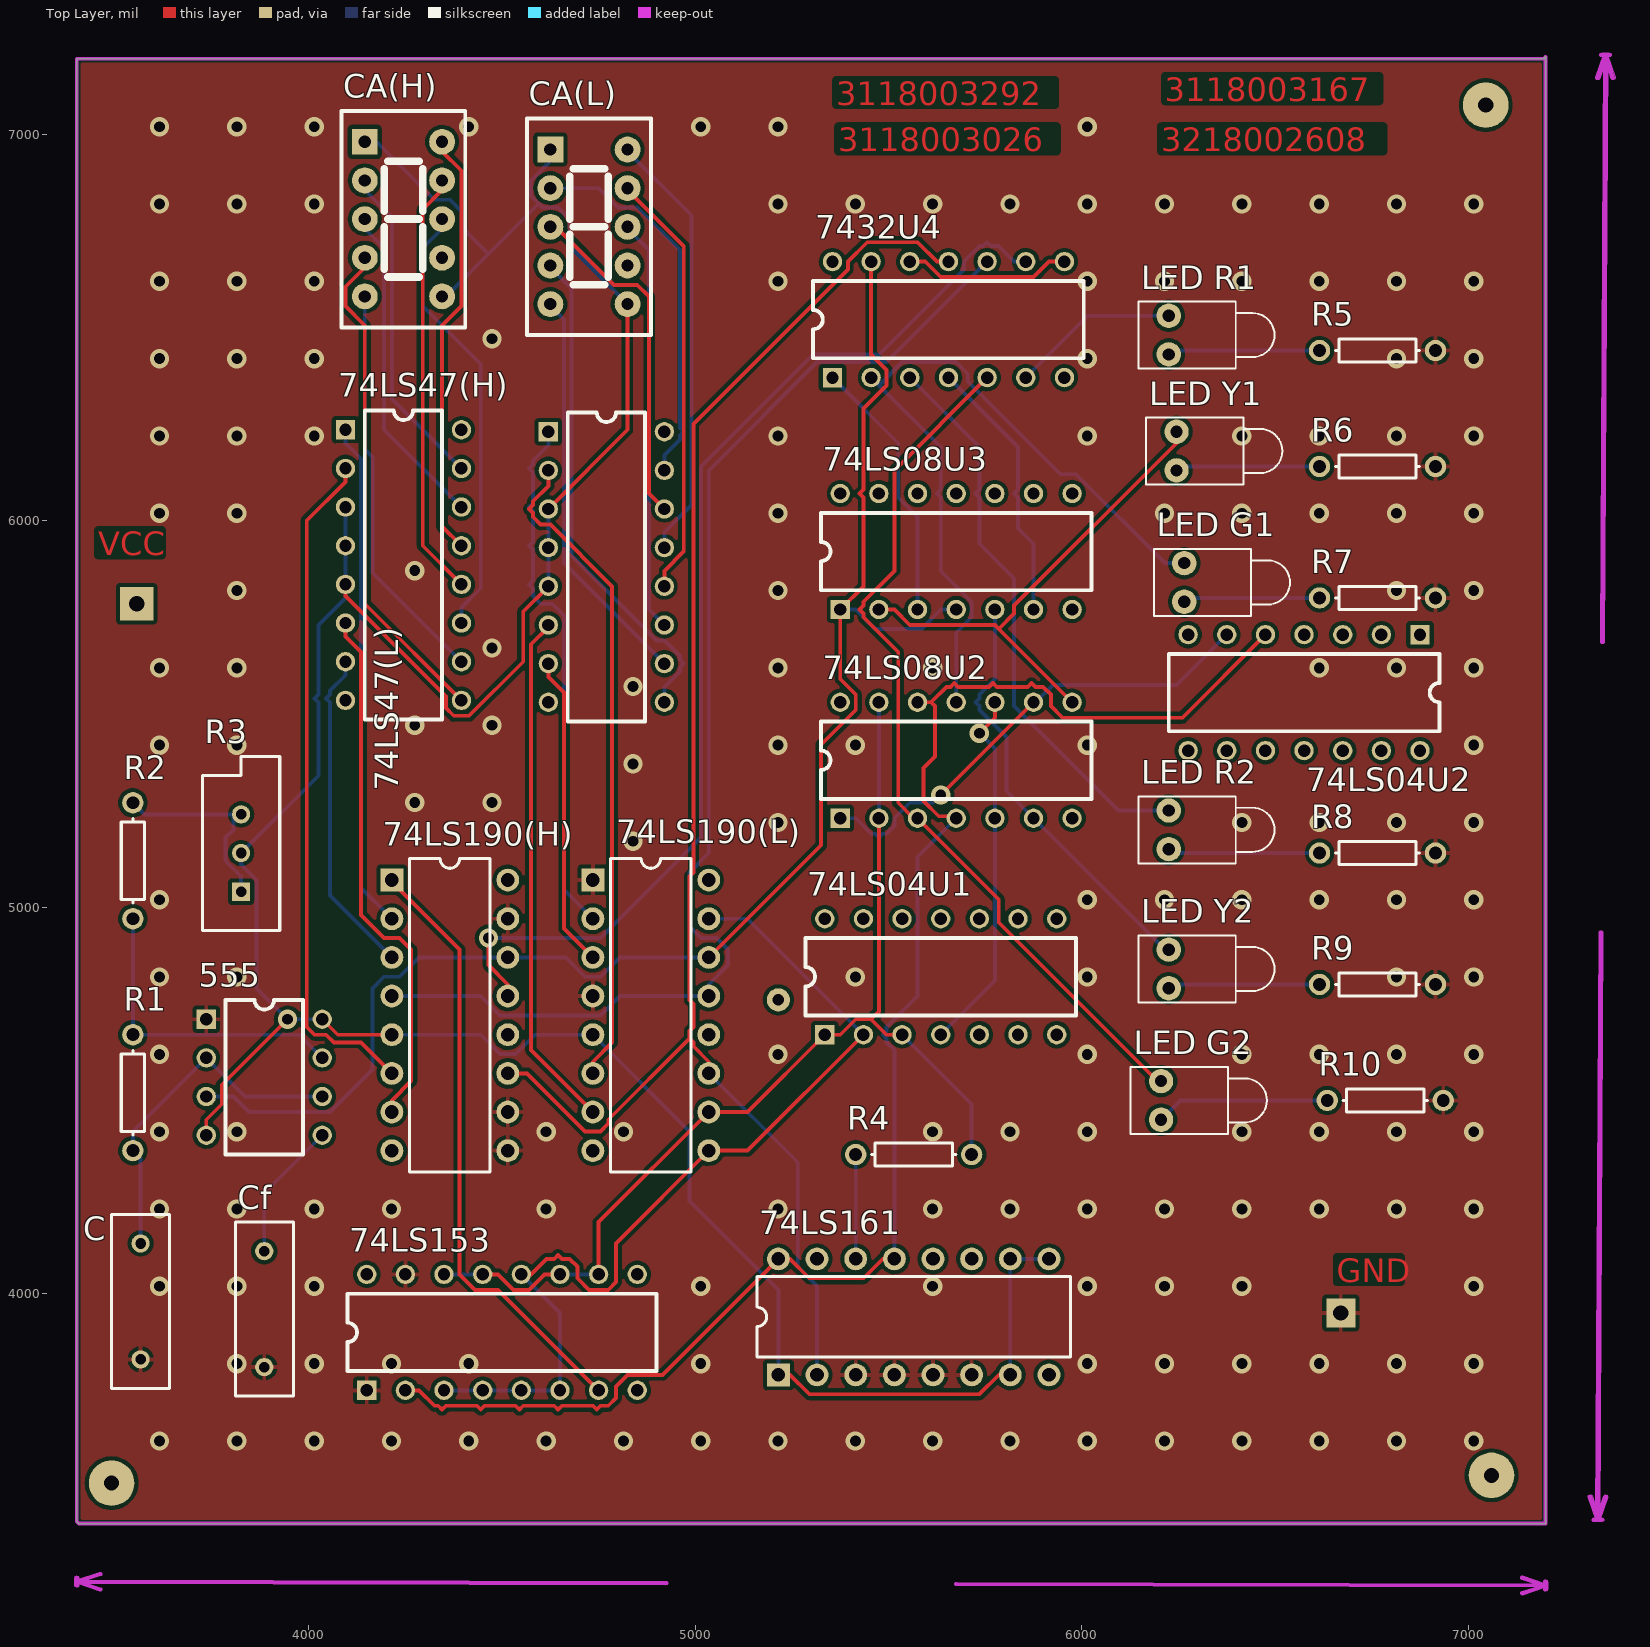
[diagram p0: Top Layer view]
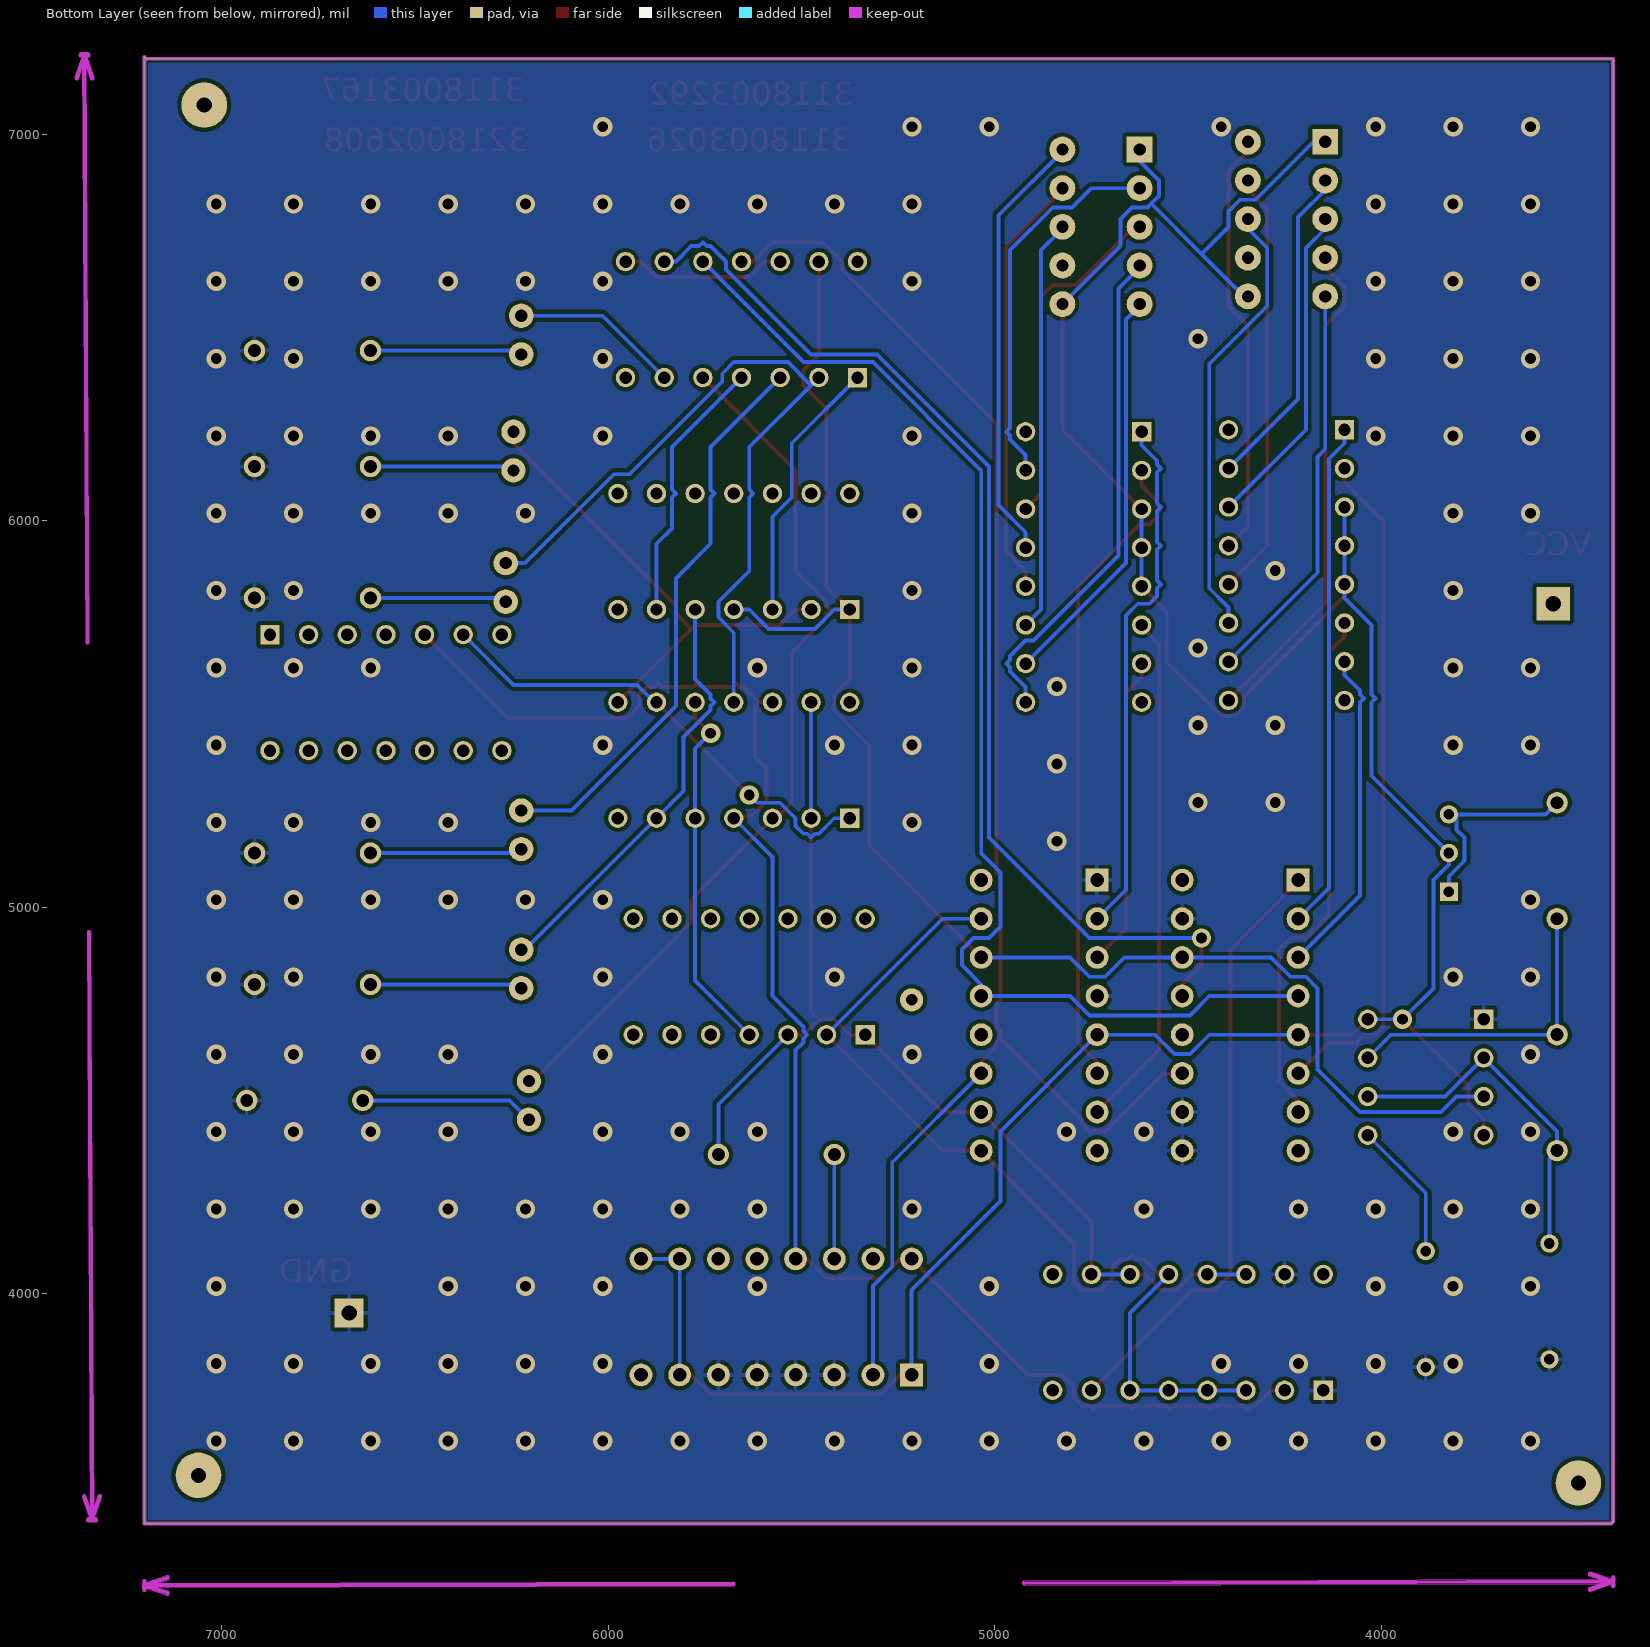
[diagram p1: Bottom Layer view, seen from below]
# Altium PCB MISC75419.pcbdoc
Units mil, origin at the board's own origin, x right, y up, seen from the top; angles counter-clockwise.
Board outline 3800 x 3795 mil, 2 copper layers (Top Layer, Bottom Layer); 32 components, 55 nets, 237 pads, 172 vias.

## Layer stack, top to bottom (the 12.6 mil dielectric is the usual default, probably not edited)
Top Solder Mask Layer: solder mask 1.4, FR-4, Dk 4.8
Top Layer: signal copper 1.4
Substrate1: surface 12.6, FR-4, Dk 4.8
Bottom Layer: signal copper 1.4
Bottom Solder Mask Layer: solder mask 1.4, FR-4, Dk 4.8

## Board outline
3400,3410 3400,7195 7195,7195 7200,7200 7200,3405 3405,3405

## Design rules (kind name [scope] priority, off if disabled: settings)
BoardOutlineClearance Plane_PlaneConnect_1 [All] p2 off: genericclearance=10 ignorepadtopadclearanceinfootprint=FALSE except(0: Arc-SplitContinuation Track-SplitContinuation SMDPad-SplitContinuation THPad-SplitContinuation Via-SplitContinuation Fill-SplitContinuation Region-SplitContinuation Poly-SplitContinuation Text-SplitContinuation Hole-SplitContinuation; 6: SMDPad-CutoutEdge THPad-CutoutEdge Via-CutoutEdge Fill-CutoutEdge Region-CutoutEdge Text-CutoutEdge; 6.9: Hole-CutoutEdge; 10: Arc-OutlineEdge Track-OutlineEdge SMDPad-OutlineEdge THPad-OutlineEdge Via-OutlineEdge Fill-OutlineEdge Region-OutlineEdge Poly-OutlineEdge Text-OutlineEdge Hole-OutlineEdge Poly-CutoutEdge; 11.8: Arc-CutoutEdge Track-CutoutEdge)
BoardOutlineClearance Copper_PolygonConnect_1 [All] p4 off: genericclearance=10 ignorepadtopadclearanceinfootprint=FALSE except(0: Arc-SplitContinuation Track-SplitContinuation SMDPad-SplitContinuation THPad-SplitContinuation Via-SplitContinuation Fill-SplitContinuation Region-SplitContinuation Poly-SplitContinuation Text-SplitContinuation Hole-SplitContinuation; 6: SMDPad-CutoutEdge THPad-CutoutEdge Via-CutoutEdge Fill-CutoutEdge Region-CutoutEdge Text-CutoutEdge; 6.9: Hole-CutoutEdge; 10: Arc-OutlineEdge Track-OutlineEdge SMDPad-OutlineEdge THPad-OutlineEdge Via-OutlineEdge Fill-OutlineEdge Region-OutlineEdge Poly-OutlineEdge Text-OutlineEdge Hole-OutlineEdge Poly-CutoutEdge; 11.8: Arc-CutoutEdge Track-CutoutEdge)
BoardOutlineClearance Clearance_1 [All] p6: genericclearance=10 ignorepadtopadclearanceinfootprint=FALSE except(0: Arc-SplitContinuation Track-SplitContinuation SMDPad-SplitContinuation THPad-SplitContinuation Via-SplitContinuation Fill-SplitContinuation Region-SplitContinuation Poly-SplitContinuation Text-SplitContinuation Hole-SplitContinuation; 6: SMDPad-CutoutEdge THPad-CutoutEdge Via-CutoutEdge Fill-CutoutEdge Region-CutoutEdge Text-CutoutEdge; 6.9: Hole-CutoutEdge; 10: Arc-OutlineEdge Track-OutlineEdge SMDPad-OutlineEdge THPad-OutlineEdge Via-OutlineEdge Fill-OutlineEdge Region-OutlineEdge Poly-OutlineEdge Text-OutlineEdge Hole-OutlineEdge Poly-CutoutEdge; 11.8: Arc-CutoutEdge Track-CutoutEdge)
Clearance Plane_PlaneConnect [All] p1 off: gap=10 ignorepadtopadclearanceinfootprint=FALSE
Clearance Copper_PolygonConnect [All] p3 off: gap=10 ignorepadtopadclearanceinfootprint=FALSE
Clearance [All] p5: gap=10 ignorepadtopadclearanceinfootprint=FALSE
DiffPairsRouting [All] p1: maxlimit=10 minlimit=10 mostfreqgap=10 toplayer_minwidth=0 toplayer_prefwidth=0 toplayer_maxwidth=0 toplayer_mingap=10 toplayer_prefgap=10 toplayer_maxgap=10 bottomlayer_minwidth=0 bottomlayer_prefwidth=0 bottomlayer_maxwidth=0 bottomlayer_mingap=10 bottomlayer_prefgap=10 bottomlayer_maxgap=10 maxuncoupledlength=10
HoleToHoleClearance ComponentClearance [All] p1: gap=10 allowstackedmicrovias=TRUE
Length netLength [All] p1: minlimit=0 maxlimit=0
PolygonConnect [(InNet('GND'))] p1: connectstyle=Relief reliefconductorwidth=10 reliefentries=4 polygonreliefangle="90 Angle" airgapwidth=10 via.connectstyle=Relief via.reliefconductorwidth=10 via.reliefentries=4 via.polygonreliefangle="90 Angle" via.airgapwidth=10
RoutingVias [All] p1: holewidth=28 width=50 viastyle="Through Hole" minholewidth=28 minwidth=50 maxholewidth=28 maxwidth=50
SolderMaskExpansion [All] p1: expansion=4 istentingtop=FALSE
Width [All] p1: maxlimit=10 minlimit=10 preferedwidth=10
2 further rules are at their usual default settings.

## Components (designator, comment, footprint, x,y, rotation, side; value= is the part's Value field where it differs from the comment)
74LS04U1 "74LS04" DIP14 5985,4720 r90 top
74LS04U2 "74LS04" DIP14 6225,5655 r270 top
74LS08U2 "74LS08" DIP14 6025,5280 r90 top
74LS08U3 "74LS08" DIP14 6025,5820 r90 top
74LS47(H) "SN7447A" DIP16 4145,5480 r0 top
74LS47(L) "SN7447A" DIP16 4670,5475 r0 top
74LS153 "SN74LS153" DIP16 4905,3800 r90 top
74LS161 "74LS161A" DIP-16 5565,3940 r0 top
74LS190(H) "SN74LS190" DIP-16 4365,4720 r270 top
74LS190(L) "SN74LS190" DIP-16 4885,4720 r270 top
555 "555" DIP8 3785,4360 r0 top
7432U4 "7432" DIP14 6005,6420 r90 top
C "Cap" RAD-0.3 3565,3980 r90 top
CA(H) "Dpy Red-CA" "SMG 0.36-1P" 4245,6780 r0 top
CA(L) "Dpy Red-CA" "SMG 0.36-1P" 4725,6760 r0 top
Cf "Cap" RAD-0.3 3885,3960 r90 top
"LED G1" "LED1" LED-1 6265,5840 r0 top
"LED G2" "LED1" LED-1 6205,4500 r0 top
"LED R1" "LED1" LED-1 6225,6480 r0 top
"LED R2" "LED1" LED-1 6225,5200 r0 top
"LED Y1" "LED1" LED-1 6245,6180 r0 top
"LED Y2" "LED1" LED-1 6225,4840 r0 top
R1 "Res1" AXIAL-0.3 3545,4520 r90 top
R2 "Res1" AXIAL-0.3 3545,5120 r90 top
R3 "RPot" VR5 3825,5140 r90 top
R4 "Res1" AXIAL-0.3 5565,4360 r180 top
R5 "Res1" AXIAL-0.3 6765,6440 r0 top
R6 "Res1" AXIAL-0.3 6765,6140 r0 top
R7 "Res1" AXIAL-0.3 6765,5800 r0 top
R8 "Res1" AXIAL-0.3 6765,5140 r0 top
R9 "Res1" AXIAL-0.3 6765,4800 r0 top
R10 "Res1" AXIAL-0.3 6785,4500 r0 top

## Footprints (in the part's own frame and the unit in brackets; to place one, negate y for a bottom-side part, rotate by r counter-clockwise, add the part's x,y. Pads: shape width x height; smd on the part's side, far side on the other; paste and mask are expansions set on the pad)
AXIAL-0.3 [mm]
  round 1.4 hole 0.85: 1(-3.81,0) 2(3.81,0)
  silkscreen extent -2.77,-0.76 2.77,0.76
DIP8 [mil]
  rect 50x50 hole 32: 1(-50,350)
  round 50 hole 32: 2(-50,250) 3(-50,150) 4(-50,50) 5(250,50) 6(250,150) 7(250,250) 8(250,350)
  silkscreen extent 0,0 200,400
DIP14 [mil]
  rect 50x50 hole 32: 1(-50,650)
  round 50 hole 32: 2(-50,550) 3(-50,450) 4(-50,350) 5(-50,250) 6(-50,150) 7(-50,50) 8(250,50) 9(250,150) 10(250,250) 11(250,350) 12(250,450) 13(250,550) 14(250,650)
  silkscreen extent 0,0 200,700
DIP16 [mil]
  rect 50x50 hole 32: 1(-50,755)
  round 50 hole 32: 2(-50,655) 3(-50,555) 4(-50,455) 5(-50,355) 6(-50,255) 7(-50,155) 8(-50,55) 9(250,55) 10(250,155) 11(250,255) 12(250,355) 13(250,455) 14(250,555) 15(250,655) 16(250,755)
  silkscreen extent 0,5 200,805
DIP-16 [mm]
  rect 1.5x1.5 hole 0.9: 1(-8.89,-3.81)
  round 1.5 hole 0.9: 2(-6.35,-3.81) 3(-3.81,-3.81) 4(-1.27,-3.81) 5(1.27,-3.81) 6(3.81,-3.81) 7(6.35,-3.81) 8(8.89,-3.81) 9(8.89,3.81) 10(6.35,3.81) 11(3.81,3.81) 12(1.27,3.81) 13(-1.27,3.81) 14(-3.81,3.81) 15(-6.35,3.81) 16(-8.89,3.81)
  silkscreen extent -10.3,-2.65 10.3,2.65
LED-1 [mm]
  round 1.6 hole 0.8: 1(0,1.27) 2(0,-1.27)
  silkscreen extent -2,-2.2 6.95,2.2
RAD-0.3 [mm]
  round 1.2 hole 0.7: 1(-3.81,0) 2(3.81,0)
  silkscreen extent -5.71,-1.91 5.71,1.91
"SMG 0.36-1P" [mm]
  rect 1.7x1.7 hole 0.8: 1(-2.54,5.08)
  round 1.7 hole 0.8: 2(-2.54,2.54) 3(-2.54,0) 4(-2.54,-2.54) 5(-2.54,-5.08) 6(2.54,-5.08) 7(2.54,-2.54) 8(2.54,0) 9(2.54,2.54) 10(2.54,5.08)
  silkscreen extent -4.06,-7.11 4.06,7.11
VR5 [mm]
  rect 1.2x1.2 hole 0.7: 1(-2.54,0)
  round 1.2 hole 0.7: 2(0,0) 3(2.54,0)
  silkscreen extent -5.08,-2.54 6.35,2.54

## Free pads (board coordinates)
  round 60 hole 30 paste+0 mask+4: 1(5215,4760)
  rect 86.61x86.61 hole 39.37 paste+0 mask+4: 2(3555,5785)
  rect 74.8x74.8 hole 39.37 paste+0 mask+4: 3(6670,3950)
  round 118.11 hole 39.37 unplated paste-1000 mask+4: 12(3490,3510) 12(7045,7075) 12(7060,3530)

## Via types
v1: diameter 50, hole 28, Top Layer to Bottom Layer, 172 vias

## Nets (pads, with @x,y where several pads share a name; then routed paths per layer and width w, separated by ;. In a path a pad name is that pad's centre, name@x,y a point inside that pad or via, vN(x,y) a via of type N, cw(c..) or ccw(c..) an arc to the next point about the centre after c; other vN are vias at no path point)
$2N11: 74LS47(H).13 CA(H).10 | length 1107.1
  Top Layer w10: 4345,6980 4345,6955 4395,6905 4395,6555 4345,6505 4345,5985 4395,5935
$2N12: 74LS47(H).12 CA(H).9 | length 1107.1
  Top Layer w10: 4345,6880 4345,6855 4295,6805 4295,5935 4395,5835
$2N13: 74LS47(H).11 CA(H).8 | length 1148.6
  Bottom Layer w10: 4345,6780 4345,6755 4295,6705 4295,6555 4445,6405 4445,5825 4395,5775 4395,5735
$2N14: 74LS47(H).10 CA(H).5 | length 1048.6
  Bottom Layer w10: 4145,6580 4145,6185 4165,6165 4165,5865 4395,5635
$2N15: 74LS47(H).9 CA(H).4 | length 1290
  Top Layer w10: 4145,6680 4145,6655 4095,6605 4095,6555 4145,6505 4145,5785 4395,5535
$2N16: 74LS47(H).15 CA(H).2 | length 848.6
  Bottom Layer w10: 4145,6880 4145,6855 4215,6785 4215,6315 4395,6135
$2N17: 74LS47(H).14 CA(H).3 | length 848.6
  Bottom Layer w10: 4145,6780 4145,6755 4195,6705 4195,6235 4395,6035
$2N18: 74LS47(L).13 CA(L).10 | length 1127.3
  Bottom Layer w10: 4825,6960 4825,6955 4990,6790 4990,6040 4920,5970 4920,5930
$2N19: 74LS47(L).12 CA(L).9 | length 1110.8
  Top Layer w10: 4825,6860 4825,6855 4970,6710 4970,5920 4920,5870 4920,5830
$2N20: 74LS47(L).11 CA(L).8 | length 1069.3
  Bottom Layer w10: 4825,6760 4825,6755 4880,6700 4880,5770 4920,5730
$2N21: 74LS47(L).10 CA(L).5 | length 1052.2
  Bottom Layer w10: 4625,6560 4625,6555 4660,6520 4660,5890 4920,5630
$2N22: 74LS47(L).9 CA(L).4 | length 1305.3
  Bottom Layer w10: 4625,6660 4625,6655 4680,6600 4680,5910 4900,5690 4920,5690 4960,5650 4960,5640 4970,5630 4960,5620 4960,5610 4920,5570 4920,5530
$2N23: 74LS47(L).15 CA(L).2 | length 996.1
  Bottom Layer w10: 4625,6860 4750,6860 4800,6810 4850,6810 4960,6700 4960,6240 4970,6230 4960,6220 4960,6210 4920,6170 4920,6130
$2N24: 74LS47(L).14 CA(L).3 | length 896.1
  Top Layer w10: 4625,6760 4640,6760 4790,6610 4850,6610 4880,6580 4880,6070 4920,6030
$2N25: 74LS47(H).6 74LS190(H).7 | length 1379.6
  Top Layer w10: 4095,5735 4095,5700 4135,5660 4135,4980 4195,4920 4235,4920 4265,4890 4265,4550 4215,4500 4215,4470
$2N26: 74LS47(H).2 74LS190(H).6 | length 1756.1
  Top Layer w10: 4095,6135 4095,6100 3995,6000 3995,4690 4015,4670 4045,4670 4065,4650 4135,4650 4215,4570
$2N27: 74LS47(H).1 74LS190(H).2 | length 1314.7
  Bottom Layer w10: 4095,6235 4095,6200 4135,6160 4135,5050 4215,4970
$2N28: 74LS47(H).7 74LS190(H).3 | length 856.1
  Bottom Layer w10: 4095,5635 4095,5600 4055,5560 4055,5550 4045,5540 4055,5530 4055,5030 4215,4870
$2N29: 74LS47(L).6 74LS190(L).7 | length 1344.9
  Top Layer w10: 4620,5730 4620,5725 4575,5680 4575,4630 4735,4470
$2N30: 74LS47(L).2 74LS190(L).6 | length 1705.1
  Top Layer w10: 4620,6130 4620,6090 4580,6050 4580,6040 4570,6030 4580,6020 4580,6010 4600,5990 4625,5990 4785,5830 4785,4650 4735,4600 4735,4570
$2N31: 74LS47(L).1 74LS190(L).2 | length 1391.5
  Bottom Layer w10: 4620,6230 4620,6195 4580,6155 4580,6145 4570,6135 4580,6125 4580,6045 4570,6035 4580,6025 4580,5945 4570,5935 4580,5925 4580,5845 4570,5835 4580,5825 4580,5805 4600,5785 4630,5785 4660,5755 4660,5045 4735,4970
$2N32: 74LS47(L).7 74LS190(L).3 | length 807.6
  Top Layer w10: 4620,5630 4620,5595 4660,5555 4660,4945 4735,4870
$2N33: 74LS190(H).13 7432U4.9 | length 2901.1
  Top Layer w10: v1(4465,4920) 4465,4850 4515,4800 4515,4770
  Bottom Layer w10: v1(4465,4920) 4755,4920 5015,5180 5015,6140 5305,6430 5475,6430 5695,6650 5695,6670 5735,6710 5745,6710 5755,6720 5765,6710 5785,6710 5825,6670 7432U4.9
$2N34: 74LS190(H).4 74LS190(L).13 7432U4.10 | length 3271.4
  Bottom Layer w10: 4215,4770 4445,4770 4495,4720 4755,4720 4805,4770 5035,4770 5035,4800 5085,4850 5085,4890 5055,4920 5015,4920 4985,4950 4985,5090 5035,5140 5035,6130 5315,6410 5495,6410 7432U4.10
$2N35: 555.5 Cf.2 | length 362.1
  Bottom Layer w10: Cf.2 3885,4260 555.5
$2N36: R2.2 R3.1 R3.3 | length 517.3
  Bottom Layer w10: R2.2 3575,5240 R3.3@3805,5240 ; R3.1 3825,5080 3785,5120 3785,5180 3805,5200 R3.3@3805,5240 ; R3.3 R3.3@3805,5240
$2N37: 555.7 R1.2 R2.1 | length 814.9
  Bottom Layer w10: R2.1 R1.2 3975,4670 555.7
$2N38: 555.2 555.6 C.2 R1.1 | length 908.4
  Bottom Layer w10: C.2 3565,4350 R1.1 3545,4420 555.2 3835,4510 555.6
$2N39: 74LS153.7 74LS190(H).1 | length 1576.7
  Top Layer w10: 4215,5070 4215,5065 4390,4890 4390,4050 4430,4010 4490,4010 74LS153.7
$2N41: 74LS161.14 R4.2 | length 270
  Bottom Layer w10: 74LS161.14 R4.2
$2N45: "LED R1.2" R5.1 | length 394.1
  Bottom Layer w10: 6225,6430 6235,6440 R5.1
$2N46: "LED Y1.2" R6.1 | length 374.1
  Bottom Layer w10: 6245,6130 6255,6140 R6.1
$2N47: "LED G1.2" R7.1 | length 354.1
  Bottom Layer w10: 6265,5790 6275,5800 R7.1
$2N48: "LED R2.2" R8.1 | length 394.1
  Bottom Layer w10: 6225,5150 6235,5140 R8.1
$2N49: "LED Y2.2" R9.1 | length 394.1
  Bottom Layer w10: 6225,4790 6235,4800 R9.1
$2N50: "LED G2.2" R10.1 | length 450.7
  Bottom Layer w10: 6205,4450 6255,4500 R10.1
$2N51: 7432U4.3 "LED R2.1" | length 1482
  Bottom Layer w10: 7432U4.3 5735,6190 5735,6080 5725,6070 5735,6060 5735,5940 5825,5850 5825,5520 6095,5250 6225,5250
$2N54: 74LS08U3.1 74LS08U3.4 74LS190(H).14 74LS190(L).14 555.3 7432U4.13 | length 4036.6
  Top Layer w10: 5035,4870 5325,5160 5325,5420 5415,5510 5415,5550 5375,5590 74LS08U3.1 5435,5830 5435,6060 5425,6070 5435,6080 5435,6290 5495,6350 5495,6390 5455,6430 7432U4.13
  Bottom Layer w10: 555.3 3805,4510 3845,4470 4055,4470 4165,4580 4165,4790 4195,4820 4235,4820 4285,4870 4515,4870 4665,4870 4715,4820 4755,4820 4805,4870 5035,4870 ; 74LS08U3.1 5415,5770 5465,5720 5585,5720 5635,5770 74LS08U3.4
$2N55: 74LS08U2.6 74LS08U3.5 "LED Y2.1" | length 1113.7
  Bottom Layer w10: 74LS08U3.5 5775,5590 5735,5550 5735,5540 5725,5530 5735,5520 5735,5510 5805,5440 5805,5300 74LS08U2.6 6215,4890 6225,4890
$2N56: 7432U4.6 "LED R1.1" | length 436.3
  Bottom Layer w10: 7432U4.6 6015,6530 6225,6530
$2N57: 74LS08U3.6 7432U4.4 | length 699.4
  Bottom Layer w10: 7432U4.4 5835,6190 5835,6080 5825,6070 5835,6060 5835,5980 5875,5940 74LS08U3.6
$2N58: 74LS08U2.3 7432U4.5 "LED G2.1" | length 2291.5
  Top Layer w10: 7432U4.5 5515,6130 5515,5870 5435,5790 5435,5780 5425,5770 5435,5760 5435,5750 5525,5660 5525,5270 5565,5230 74LS08U2.3 5785,5020 5785,4960 6195,4550 6205,4550
$2N62: 7432U4.8 7432U4.12 | length 433.1
  Top Layer w10: 7432U4.12 5595,6670 5635,6630 5875,6630 5915,6670 7432U4.8
$2N63: 74LS161.2 74LS190(H).11 74LS190(L).11 7432U4.11 | length 4133.6
  Top Layer w10: 4515,4570 4565,4570 4715,4420 4755,4420 4775,4440 4775,4450 4985,4660 ; 5035,4570 5035,4600 4995,4640 4995,4650 4985,4660 ; 7432U4.11 5625,6670 5575,6720 5445,6720 5395,6670 5395,6650 4995,6250 4995,5090 4985,5080 4985,4760 4995,4750 4995,4690 4985,4680 4985,4660
  Bottom Layer w10: 5035,4570 5265,4340 5265,4070 5315,4020 74LS161.2
$2N1237: 74LS08U3.3 7432U4.1 | length 691.1
  Bottom Layer w10: 7432U4.1 5525,6200 5525,6060 5575,6010 74LS08U3.3
$2N1241: 74LS08U2.11 7432U4.2 "LED G1.1" | length 2014.5
  Bottom Layer w10: 7432U4.2 5475,6350 ; 74LS08U2.11 5675,5710 5715,5750 5715,5790 5635,5870 5635,6060 5625,6070 5635,6080 5635,6190 5475,6350 ; 6265,5890 6215,5890 5985,6120 5945,6120 5705,6360 5705,6380 5675,6410 5535,6410 5475,6350
$2N1342: 74LS04U1.4 74LS08U2.5 74LS08U2.10 | length 951.1
  Top Layer w10: v1(5735,5450) 5775,5490 74LS08U2.10
  Bottom Layer w10: 74LS04U1.4 5775,4810 74LS08U2.5 5775,5410 v1(5735,5450)
$2N1374: 74LS04U2.5 74LS08U2.4 74LS08U2.12 74LS153.2 74LS161.13 74LS161.16 | length 4226.9
  Top Layer w10: 74LS153.2 4285,3750 4325,3710 4335,3710 4345,3700 4355,3710 4435,3710 4445,3700 4455,3710 4535,3710 4545,3700 4555,3710 4635,3710 4645,3700 4655,3710 4735,3710 4745,3700 4755,3710 4775,3710 4795,3730 4795,3760 4825,3790 4915,3790 74LS161.16 5245,4090 5295,4040 5435,4040 5485,4090 74LS161.13 ; 74LS08U2.12 5610,5530 ; 74LS08U2.4 5670,5235 5630,5235 5590,5275 5590,5360 5620,5390 5620,5520 5610,5530 ; 74LS04U2.5 6259.99,5490 5949.99,5490 5919.99,5520 5919.99,5550 5899.99,5570 5880,5570 5870,5580 5860,5570 5780,5570 5770,5580 5760,5570 5680,5570 5670,5580 5660,5570 5650,5570 5610,5530
  Bottom Layer w10: 74LS161.13 5515,4630 5495,4650 5495,4660 5485,4670 5495,4680 5495,4690 5575,4770 5575,5130 74LS08U2.4
$2N1447: 74LS04U2.6 74LS08U2.1 74LS08U2.9 | length 1249.9
  Top Layer w10: v1(5635,5290) 74LS08U2.9
  Bottom Layer w10: 74LS08U2.1 5415,5230 5455,5190 5465,5190 5475,5180 5485,5190 5495,5190 5515,5210 5515,5230 5555,5270 5615,5270 v1(5635,5290) ; 74LS08U2.9 5880,5530 5925,5575 6245,5575 74LS04U2.6
$2N1530: 74LS08U2.8 74LS08U3.2 "LED Y1.1" | length 1300
  Top Layer w10: 74LS08U3.2 5515,5770 5555,5730 5775,5730 5785,5720 ; 74LS08U2.8 5785,5720 ; 6245,6230 6245,6200 5825,5780 5825,5760 5785,5720
$2N1733: 74LS04U1.2 74LS153.3 74LS153.4 74LS153.5 74LS153.6 74LS153.12 74LS190(L).9 74LS190(L).15 | length 2458.2
  Top Layer w10: 74LS153.12 4575,4050 4615,4090 4635,4090 4645,4100 4655,4090 4675,4090 4695,4070 4695,4040 4725,4010 4775,4010 4795,4030 4795,4130 5035,4370 5135,4370 74LS04U1.2
  Bottom Layer w10: 74LS153.3 74LS153.4 74LS153.5 74LS153.6 4650,3950 74LS153.12 ; 5035,4970 5135,4970 74LS04U1.2
$2N2029: 74LS04U1.1 74LS04U1.3 74LS08U2.2 74LS08U2.13 74LS153.10 74LS153.11 74LS153.13 74LS153.14 74LS190(L).10 R4.1 | length 2800
  Top Layer w10: 74LS153.13 4490,4050 4530,4010 4570,4010 4610,4050 74LS153.11 ; 74LS153.10 4750,4185 5035,4470 5135,4470 74LS04U1.1 5375,4670 5415,4710 5455,4710 ; 74LS08U2.2 5475,4730 5455,4710 ; 74LS04U1.3 5495,4670 5455,4710
  Bottom Layer w10: 74LS153.14 74LS153.13 ; 74LS153.11 74LS153.10 ; 74LS08U2.2 74LS08U2.13 ; 74LS04U1.3 5715,4490 R4.1
+5: 74LS47(H).3 74LS47(H).4 74LS47(H).5 74LS47(L).3 74LS47(L).4 74LS47(L).5 74LS161.1 74LS161.7 74LS161.9 74LS161.10 74LS190(H).5 74LS190(L).5 555.4 555.8 CA(H).1 CA(H).6 CA(L).1 CA(L).6 R3.2 | length 7941.5
  Top Layer w10: 555.4 3735,4450 3775,4490 3775,4540 v1(3945,4710) ; 555.8 4075,4670 4215,4670 ; 4095,5835 4095,5805 4355,5545 4355,5515 4375,5495 4415,5495 4555,5635 4555,5765.05 4620,5830 ; 4620,6030 4825,6235 4825,6560 ; 74LS161.1 5245,3790 5295,3740 5735,3740 5785,3790 74LS161.7
  Bottom Layer w10: 555.8 v1(3945,4710) 3865,4790 3865,5070 3825,5110 R3.2 4025,5340 4025,5530 4015,5540 4025,5550 4025,5730 4095,5800 4095,5835 4095,5935 4095,6035 ; 4145,6980 4175,6980 4325,6830 4365,6830 4395,6800 4395,6760 4465,6690 ; 4215,4670 4445,4670 4495,4620 4535,4620 4585,4670 4735,4670 4985,4420 4985,4240 5215,4010 74LS161.1 ; 4345,6580 4355,6580 4465,6690 ; 4620,5830 4620,5930 4620,6030 ; 4625,6960 4625,6930 4575,6880 4575,6840 4595,6820 ; 4825,6560 4675,6710 4675,6780 4645,6810 4605,6810 4595,6820 ; 74LS161.7 74LS161.10 74LS161.9 ; 4465,6690 4595,6820
GND: 74LS153.1 74LS153.15 74LS161.3 74LS161.4 74LS161.5 74LS161.6 74LS190(H).9 74LS190(H).10 74LS190(H).15 74LS190(L).1 74LS190(L).4 555.1 C.1 Cf.1 pad.3 R5.2 R6.2 R7.2 R8.2 R9.2 R10.2
  other v1: 3614.1,3619.1 3814.1,3619.1 4014.1,3619.1 4214.1,3619.1 4414.1,3619.1 4614.1,3619.1 4814.1,3619.1 5014.1,3619.1 5214.1,3619.1 5414.1,3619.1 5614.1,3619.1 5814.1,3619.1 6014.1,3619.1 6214.1,3619.1 6414.1,3619.1 6614.1,3619.1 6814.1,3619.1 7014.1,3619.1 3814.1,3819.1 4014.1,3819.1 4214.1,3819.1 4414.1,3819.1 5014.1,3819.1 6014.1,3819.1 6214.1,3819.1 6414.1,3819.1 6614.1,3819.1 6814.1,3819.1 7014.1,3819.1 3614.1,4019.1 3814.1,4019.1 4014.1,4019.1 5014.1,4019.1 5614.1,4019.1 6014.1,4019.1 6214.1,4019.1 6414.1,4019.1 7014.1,4019.1 3614.1,4219.1 3814.1,4219.1 4014.1,4219.1 4214.1,4219.1 4614.1,4219.1 5214.1,4219.1 5614.1,4219.1 5814.1,4219.1 6014.1,4219.1 6214.1,4219.1 6414.1,4219.1 6614.1,4219.1 6814.1,4219.1 7014.1,4219.1 3614.1,4419.1 3814.1,4419.1 4614.1,4419.1 4814.1,4419.1 5614.1,4419.1 5814.1,4419.1 6014.1,4419.1 6414.1,4419.1 6614.1,4419.1 6814.1,4419.1 7014.1,4419.1 3614.1,4619.1 5214.1,4619.1 6014.1,4619.1 6414.1,4619.1 6614.1,4619.1 6814.1,4619.1 7014.1,4619.1 3614.1,4819.1 3814.1,4819.1 5414.1,4819.1 6014.1,4819.1 6814.1,4819.1 7014.1,4819.1 3614.1,5019.1 6014.1,5019.1 6214.1,5019.1 6414.1,5019.1 6614.1,5019.1 6814.1,5019.1 7014.1,5019.1 4839.1,5170.64 5214.1,5219.1 6414.1,5219.1 6614.1,5219.1 6814.1,5219.1 7014.1,5219.1 4274.1,5270.64 4474.1,5270.64 4839.1,5370.64 3614.1,5419.1 3814.1,5419.1 5214.1,5419.1 5414.1,5419.1 6014.1,5419.1 7014.1,5419.1 4274.1,5470.64 4474.1,5470.64 4839.1,5570.64 3614.1,5619.1 3814.1,5619.1 5214.1,5619.1 5614.1,5619.1 6614.1,5619.1 6814.1,5619.1 7014.1,5619.1 4474.1,5670.64 3814.1,5819.1 5214.1,5819.1 6814.1,5819.1 7014.1,5819.1 4274.1,5870.64 3614.1,6019.1 3814.1,6019.1 5214.1,6019.1 6214.1,6019.1 6414.1,6019.1 6614.1,6019.1 6814.1,6019.1 7014.1,6019.1 3614.1,6219.1 3814.1,6219.1 4014.1,6219.1 5214.1,6219.1 6014.1,6219.1 6414.1,6219.1 6614.1,6219.1 6814.1,6219.1 7014.1,6219.1 3614.1,6419.1 3814.1,6419.1 4014.1,6419.1 6014.1,6419.1 6814.1,6419.1 7014.1,6419.1 4474.1,6470.64 3614.1,6619.1 3814.1,6619.1 4014.1,6619.1 5214.1,6619.1 6014.1,6619.1 6214.1,6619.1 6414.1,6619.1 6614.1,6619.1 6814.1,6619.1 7014.1,6619.1 3614.1,6819.1 3814.1,6819.1 4014.1,6819.1 5214.1,6819.1 5414.1,6819.1 5614.1,6819.1 5814.1,6819.1 6014.1,6819.1 6214.1,6819.1 6414.1,6819.1 6614.1,6819.1 6814.1,6819.1 7014.1,6819.1 3614.1,7019.1 3814.1,7019.1 4014.1,7019.1 4414.1,7019.1 5014.1,7019.1 5214.1,7019.1 6014.1,7019.1
VCC: pad.1
pads on no net: 74LS04U1.5 74LS04U1.6 74LS04U1.7 74LS04U1.8 74LS04U1.9 74LS04U1.10 74LS04U1.11 74LS04U1.12 74LS04U1.13 74LS04U1.14 74LS04U2.1 74LS04U2.2 74LS04U2.3 74LS04U2.4 74LS04U2.7 74LS04U2.8 74LS04U2.9 74LS04U2.10 74LS04U2.11 74LS04U2.12 74LS04U2.13 74LS04U2.14 74LS08U2.7 74LS08U2.14 74LS08U3.7 74LS08U3.8 74LS08U3.9 74LS08U3.10 74LS08U3.11 74LS08U3.12 74LS08U3.13 74LS08U3.14 74LS47(H).8 74LS47(H).16 74LS47(L).8 74LS47(L).16 74LS153.8 74LS153.9 74LS153.16 74LS161.8 74LS161.11 74LS161.12 74LS161.15 74LS190(H).8 74LS190(H).12 74LS190(H).16 74LS190(L).8 74LS190(L).12 74LS190(L).16 7432U4.7 7432U4.14 CA(H).7 CA(L).7

## Polygon pours and split planes (outlines as drawn)
GND on Top Layer (solid, remove dead copper, pour order 0): 3000,7555 3000,3225 8280,3225 8280,7555
GND on Bottom Layer (solid, remove dead copper, pour order 2): 3075,7555 3075,3000 7635,3000 7635,7555

## Keep-outs
Board Outline Layer:
  region: 7370,7204.95 7369.62,7203.03 7368.54,7201.41 7366.91,7200.33 7365,7199.95 7364.97,7199.95 7344.97,7200.05 7343.07,7200.44 7341.46,7201.53 7340.38,7203.15 7340,7205.05 7340.38,7206.97 7341.46,7208.59 7343.09,7209.67 7345,7210.05 7345.03,7210.05 7365.03,7209.95 7366.93,7209.56 7368.54,7208.47 7369.62,7206.85
  region: 7350,3414.95 7349.62,3413.03 7348.54,3411.41 7346.91,3410.33 7345,3409.95 7344.97,3409.95 7324.97,3410.05 7323.07,3410.44 7321.46,3411.53 7320.38,3413.15 7320,3415.05 7320.38,3416.97 7321.46,3418.59 7323.09,3419.67 7325,3420.05 7325.03,3420.05 7345.03,3419.95 7346.93,3419.56 7348.54,3418.47 7349.62,3416.85 7350,3414.95
  region: 7374.68,7139.9 7373.14,7140.14 7371.75,7140.85 7370.64,7141.95 7369.93,7143.34 7354.92,7189.19 7339.42,7143.5 7338.7,7142.13 7337.6,7141.04 7336.21,7140.35 7334.68,7140.11 7332.77,7140.49 7331.15,7141.57 7330.06,7143.19 7329.68,7145.11 7329.75,7145.92 7329.95,7146.71 7350.27,7206.61 7350.98,7207.98 7352.09,7209.06 7353.47,7209.76 7355,7210 7356.54,7209.76 7357.93,7209.05 7359.04,7207.95 7359.75,7206.56 7379.43,7146.45 7379.62,7145.68 7379.68,7144.9 7379.3,7142.98 7378.22,7141.36 7376.6,7140.28
  region: 7335,3410 7333.46,3410.24 7332.07,3410.95 7330.96,3412.05 7330.25,3413.44 7310.57,3473.55 7310.38,3474.32 7310.32,3475.1 7310.7,3477.02 7311.78,3478.64 7313.4,3479.72 7315.32,3480.1 7316.86,3479.86 7318.25,3479.15 7319.36,3478.05 7320.07,3476.66 7335.08,3430.81 7350.58,3476.5 7351.3,3477.87 7352.4,3478.96 7353.79,3479.65 7355.32,3479.89 7357.23,3479.51 7358.85,3478.43 7359.94,3476.81 7360.32,3474.89 7360.25,3474.08 7360.05,3473.29 7339.73,3413.39 7339.02,3412.02 7337.91,3410.94 7336.53,3410.24
  region: 7351.98,5685.85 7351.6,5683.95 7350.51,5682.33 7348.89,5681.26 7346.98,5680.88 7345.07,5681.26 7343.45,5682.34 7342.36,5683.97 7341.98,5685.88 7341.98,5685.9 7350,7205.03 7350.39,7206.93 7351.47,7208.54 7353.09,7209.62 7355,7210 7356.91,7209.62 7358.54,7208.54 7359.62,7206.91 7360,7205 7360,7204.97 7351.98,5685.85
  region: 7340,3414.97 7339.61,3413.07 7338.53,3411.46 7336.91,3410.38 7335,3410 7333.09,3410.38 7331.46,3411.46 7330.38,3413.09 7330,3415 7330,3415.03 7338.02,4934.15 7338.4,4936.05 7339.49,4937.67 7341.11,4938.74 7343.02,4939.12 7344.93,4938.74 7346.55,4937.66 7347.64,4936.03 7348.02,4934.12 7348.02,4934.1 7340,3414.97
  region: 7204.97,3234.99 7204.59,3233.08 7203.5,3231.46 7201.88,3230.38 7199.97,3230 7198.06,3230.38 7196.44,3231.46 7195.35,3233.09 7194.97,3235 7194.97,3235.01 7195.03,3255.01 7195.41,3256.92 7196.5,3258.54 7198.12,3259.62 7200.03,3260 7201.94,3259.62 7203.56,3258.54 7204.65,3256.91 7205.03,3255 7205.03,3254.99 7204.97,3234.99
  region: 3404.97,3244.99 3404.59,3243.08 3403.5,3241.46 3401.88,3240.38 3399.97,3240 3398.06,3240.38 3396.44,3241.46 3395.35,3243.09 3394.97,3245 3394.97,3245.01 3395.03,3265.01 3395.41,3266.92 3396.5,3268.54 3398.12,3269.62 3400.03,3270 3401.94,3269.62 3403.56,3268.54 3404.65,3266.91 3405.03,3265 3405.03,3264.99 3404.97,3244.99
  region: 7141.52,3220.41 7140.74,3220.22 7139.95,3220.16 7138.03,3220.54 7136.41,3221.62 7135.33,3223.24 7134.95,3225.16 7135.19,3226.7 7135.9,3228.09 7136.99,3229.19 7138.38,3229.91 7184.19,3245.04 7138.46,3260.42 7137.08,3261.14 7135.99,3262.24 7135.29,3263.62 7135.05,3265.16 7135.43,3267.07 7136.52,3268.69 7138.14,3269.78 7140.05,3270.16 7140.86,3270.09 7141.65,3269.9 7201.59,3249.74 7202.97,3249.02 7204.06,3247.92 7204.76,3246.53 7205,3245 7204.76,3243.46 7204.05,3242.07 7202.95,3240.97 7201.57,3240.25 7141.52,3220.41
  region: 3464.95,3234.84 3464.57,3232.93 3463.48,3231.31 3461.86,3230.22 3459.95,3229.84 3459.14,3229.91 3458.35,3230.1 3398.41,3250.26 3397.03,3250.98 3395.94,3252.08 3395.24,3253.47 3395,3255 3395.24,3256.54 3395.95,3257.93 3397.05,3259.03 3398.43,3259.75 3458.48,3279.59 3459.26,3279.78 3460.05,3279.84 3461.97,3279.46 3463.59,3278.38 3464.67,3276.76 3465.05,3274.84 3464.81,3273.3 3464.1,3271.91 3463.01,3270.81 3461.62,3270.09 3415.81,3254.96 3461.54,3239.58 3462.92,3238.86 3464.01,3237.76 3464.71,3236.38 3464.95,3234.84
  region: 7205,3245 7204.62,3243.09 7203.54,3241.46 7201.91,3240.38 7200,3240 7199.99,3240 5675.87,3244.01 5673.96,3244.4 5672.34,3245.48 5671.26,3247.1 5670.88,3249.01 5671.26,3250.92 5672.35,3252.55 5673.97,3253.63 5675.88,3254.01 5675.9,3254.01 7200.01,3250 7201.92,3249.62 7203.54,3248.53 7204.62,3246.91
  region: 4929.12,3250.99 4928.74,3249.08 4927.65,3247.45 4926.03,3246.37 4924.12,3245.99 4924.1,3245.99 3399.99,3250 3398.08,3250.38 3396.46,3251.47 3395.38,3253.09 3395,3255 3395.38,3256.91 3396.46,3258.54 3398.09,3259.62 3400,3260 3400.01,3260 4924.13,3255.99 4926.04,3255.6 4927.66,3254.52 4928.74,3252.9 4929.12,3250.99
  lines w10: 3399.97,3245 3400.03,3265 ; 3459.95,3234.84 3400,3255 ; 3460.05,3274.84 3400,3255 ; 4924.12,3250.99 3400,3255 ; 5675.88,3249.01 7200,3245 ; 7139.95,3225.16 7200,3245 ; 7140.05,3265.16 7200,3245 ; 7199.97,3235 7200.03,3255 ; 7315.32,3475.1 7335,3415 ; 7325,3415.05 7345,3414.95 ; 7334.68,7145.11 7355,7205 ; 7343.02,4934.12 7335,3415 ; 7345,7205.05 7365,7204.95 ; 7346.98,5685.88 7355,7205 ; 7355.32,3474.89 7335,3415 ; 7374.68,7144.9 7355,7205 ; 3400,3410 3400,7195 7195,7195 7200,7200 7200,3405 3405,3405 3400,3410
  text "96.26734 (mm)" at 7379.06,4943.93 h60 r89.7
  text "96.52034 (mm)" at 4934.02,3214.97 h60 r359.8

## Other copper
Top Layer:
  text "3118003167" at 6215,7085 h60
  text "3118003292" at 5365,7075 h60
  text "3118003026" at 5370,6955 h60
  text "3218002608" at 6205,6955 h60
  text "VCC" at 3455,5910 h60
  text "GND" at 6660,4030 h60

## Dimensions
7335,3415 to 7355,7205 on Board Outline Layer
3400,3255 to 7200,3245 on Board Outline Layer